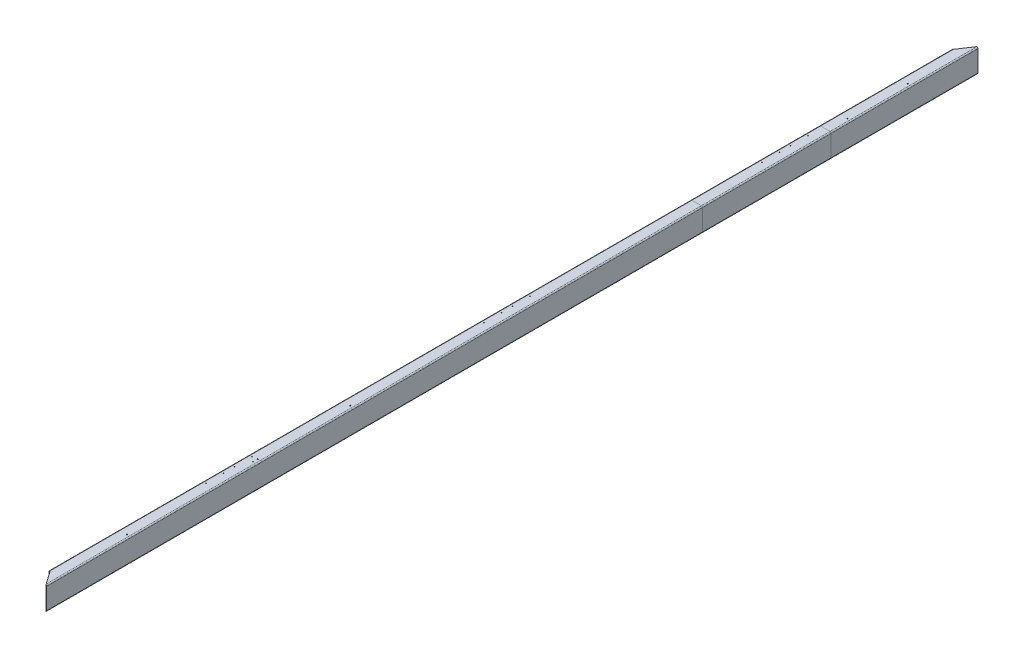
SolidWorks part; units mm, degrees
ref_plane "前视基准面" through (0, 0, 0) normal (0, 0, 1) x (1, 0, 0)
ref_plane "上视基准面" through (0, 0, 0) normal (0, 1, 0) x (1, 0, 0)
ref_plane "右视基准面" through (0, 0, 0) normal (1, 0, 0) x (0, 0, -1)
sketch "草图1" plane through (0, 0, 0) normal (0, 0, 1) x (1, 0, 0)
  line L1 (-20, 50) -> (20, 50)
  line L2 (-25, 45) -> (-25, -45)
  line L3 (-20, -50) -> (20, -50)
  line L4 (25, 45) -> (25, -45)
  line L5 (-25, 50) -> (25, -50) construction
  line L6 (-25, -50) -> (25, 50) construction
  arc A0 (20, -50) -> (25, -45) centre (20, -45) ccw
  arc A1 (-25, -45) -> (-20, -50) centre (-20, -45) ccw
  arc A2 (20, 50) -> (25, 45) centre (20, 45) cw
  arc A3 (-20, 50) -> (-25, 45) centre (-20, 45) ccw
  point P0 (0, 0)
  dimension "D3" = 5
  dimension "D1" = 50
  dimension "D2" = 100
extrude "拉伸-薄壁1" add sketch "草图1" along normal mid plane 2754 thin
sketch "草图2" plane through (0, 0, 1377) normal (0, 0, 1) x (1, 0, 0)
  line L0 (-20, -50) -> (20, -50) construction
  line L1 (-20, -46) -> (20, -46) construction
  line L2 (21, -45) -> (21, 45) construction
  line L3 (25, -45) -> (25, 45) construction
  line L4 (-21, 45) -> (-21, -45) construction
  line L5 (-25, 45) -> (-25, -45) construction
  line L6 (20, 46) -> (-20, 46) construction
  line L7 (20, 50) -> (-20, 50) construction
  line L8 (-20, -50) -> (20, -50)
  line L9 (-20, -46) -> (20, -46)
  line L10 (21, -45) -> (21, 45)
  line L11 (25, -45) -> (25, 45)
  line L12 (-21, 45) -> (-21, -45)
  line L13 (-25, 45) -> (-25, -45)
  line L14 (20, 46) -> (-20, 46)
  line L15 (20, 50) -> (-20, 50)
  arc A0 (20, -50) -> (25, -45) centre (20, -45) ccw construction
  arc A1 (20, -46) -> (21, -45) centre (20, -45) ccw construction
  arc A2 (-25, -45) -> (-20, -50) centre (-20, -45) ccw construction
  arc A3 (-21, -45) -> (-20, -46) centre (-20, -45) ccw construction
  arc A4 (21, 45) -> (20, 46) centre (20, 45) ccw construction
  arc A5 (-20, 46) -> (-21, 45) centre (-20, 45) ccw construction
  arc A6 (25, 45) -> (20, 50) centre (20, 45) ccw construction
  arc A7 (-20, 50) -> (-25, 45) centre (-20, 45) ccw construction
  arc A8 (20, -50) -> (25, -45) centre (20, -45) ccw
  arc A9 (20, -46) -> (21, -45) centre (20, -45) ccw
  arc A10 (-25, -45) -> (-20, -50) centre (-20, -45) ccw
  arc A11 (-21, -45) -> (-20, -46) centre (-20, -45) ccw
  arc A12 (21, 45) -> (20, 46) centre (20, 45) ccw
  arc A13 (-20, 46) -> (-21, 45) centre (-20, 45) ccw
  arc A14 (25, 45) -> (20, 50) centre (20, 45) ccw
  arc A15 (-20, 50) -> (-25, 45) centre (-20, 45) ccw
extrude "凸台-拉伸1" add sketch "草图2" along normal blind 60 separate body
sketch "草图3" plane through (0, 50, 0) normal (0, 1, 0) x (1, 0, 0)
  line L0 (-20, -1377) -> (22.0125, -1437)
  line L2 (20, -1377) -> (-20, -1377) construction
  line L3 (-20, -1377) -> (-44.1333, -1377)
  line L4 (-44.1333, -1377) -> (-44.1333, -1437)
  line L5 (-44.1333, -1437) -> (22.0125, -1437)
  line L6 (20, -1437) -> (-20, -1437) construction
  line L7 (20, -1437) -> (25, -1437) construction
  dimension "D1" = 55
extrude "切除-拉伸1" cut sketch "草图3" against normal through all
sketch "草图4" plane through (0, 0, -1377) normal (0, 0, -1) x (-1, 0, 0)
  line L0 (20, -46) -> (-20, -46) construction
  line L1 (20, -50) -> (-20, -50) construction
  line L2 (-21, -45) -> (-21, 45) construction
  line L3 (-25, -45) -> (-25, 45) construction
  line L4 (25, 45) -> (25, -45) construction
  line L5 (21, 45) -> (21, -45) construction
  line L6 (-20, 46) -> (20, 46) construction
  line L7 (-20, 50) -> (20, 50) construction
  line L8 (20, -46) -> (-20, -46)
  line L9 (20, -50) -> (-20, -50)
  line L10 (-21, -45) -> (-21, 45)
  line L11 (-25, -45) -> (-25, 45)
  line L12 (25, 45) -> (25, -45)
  line L13 (21, 45) -> (21, -45)
  line L14 (-20, 46) -> (20, 46)
  line L15 (-20, 50) -> (20, 50)
  arc A0 (-25, -45) -> (-20, -50) centre (-20, -45) ccw construction
  arc A1 (-21, -45) -> (-20, -46) centre (-20, -45) ccw construction
  arc A2 (20, -46) -> (21, -45) centre (20, -45) ccw construction
  arc A3 (20, -50) -> (25, -45) centre (20, -45) ccw construction
  arc A4 (21, 45) -> (20, 46) centre (20, 45) ccw construction
  arc A5 (25, 45) -> (20, 50) centre (20, 45) ccw construction
  arc A6 (-20, 46) -> (-21, 45) centre (-20, 45) ccw construction
  arc A7 (-20, 50) -> (-25, 45) centre (-20, 45) ccw construction
  arc A8 (-25, -45) -> (-20, -50) centre (-20, -45) ccw
  arc A9 (-21, -45) -> (-20, -46) centre (-20, -45) ccw
  arc A10 (20, -46) -> (21, -45) centre (20, -45) ccw
  arc A11 (20, -50) -> (25, -45) centre (20, -45) ccw
  arc A12 (21, 45) -> (20, 46) centre (20, 45) ccw
  arc A13 (25, 45) -> (20, 50) centre (20, 45) ccw
  arc A14 (-20, 46) -> (-21, 45) centre (-20, 45) ccw
  arc A15 (-20, 50) -> (-25, 45) centre (-20, 45) ccw
extrude "凸台-拉伸2" add sketch "草图4" along normal blind 1182 separate body
sketch "草图5" plane through (0, 50, 0) normal (0, 1, 0) x (1, 0, 0)
  line L0 (20, 2559) -> (-20, 2499)
  line L1 (-20, 2559) -> (-20, 1377) construction
  line L2 (-20, 2559) -> (20, 2559) construction
  line L3 (-20, 2499) -> (-29.878, 2499)
  line L4 (-29.878, 2499) -> (-29.878, 2930.2275)
  line L5 (-29.878, 2930.2275) -> (20, 2930.2275)
  line L6 (20, 2930.2275) -> (20, 2559)
  dimension "D1" = 60
extrude "切除-拉伸2" cut sketch "草图5" against normal through all
sketch "草图6" plane through (0, 50, 0) normal (0, 1, 0) x (1, 0, 0)
  line L0 (-353.4481, 1929) -> (237.5908, 1929)
  line L1 (25, 2559) -> (20, 2559) construction
  dimension "D1" = 630
split line "分割线1"
hole_wizard "M3 螺纹孔1" positions "草图9" profile "草图8" tap size "M3" standard "GB"
sketch "草图9" plane through (0, 50, 0) normal (0, 1, 0) x (1, 0, 0)
  line L1 (-8.25, -717) -> (-13.75, -717) construction
  line L3 (-13.75, -642) -> (-8.25, -642) construction
  line L5 (-13.75, -594.5) -> (-8.25, -594.5) construction
  line L8 (-13.75, -519.5) -> (-8.25, -519.5) construction
  line L10 (-11, -1519.5) -> (-11, 48480.5) construction
  line L11 (-8.25, 476) -> (-11, 476) construction
  line L13 (-8.25, 551) -> (-11, 551) construction
  line L15 (-8.25, 597.5) -> (-11, 597.5) construction
  line L17 (-8.25, 672.5) -> (-11, 672.5) construction
  line L19 (-8.25, 1743) -> (-11, 1743) construction
  line L21 (-8.25, 1668) -> (-11, 1668) construction
  line L23 (-8.25, 1790.5) -> (-11, 1790.5) construction
  line L25 (-8.25, 1865.5) -> (-11, 1865.5) construction
  point P28 (-11, -642)
  point P30 (-11, -717)
  point P32 (-11, -594.5)
  point P34 (-11, -519.5)
  point P44 (-11, 476)
  point P49 (-11, 551)
  point P54 (-11, 597.5)
  point P59 (-11, 672.5)
  point P63 (-11, 1743)
  point P68 (-11, 1668)
  point P72 (-11, 1790.5)
  point P77 (-11, 1865.5)
sketch "草图8" plane through (-11, 50, -1865.5) normal (1, 0, 0) x (0, 0, 1)
  line L0 (0, 0) -> (0, 9.2511)
  line L1 (0, 9.2511) -> (1.25, 8.5)
  line L2 (1.25, 8.5) -> (1.25, 0.275)
  line L3 (1.25, 0.275) -> (1.525, 0)
  line L5 (1.525, 0) -> (0, 0)
  line L6 (-1.25, 0.275) -> (-1.525, 0) construction
  line L10 (0, 9.2511) -> (-1.25, 8.5) construction
  line L11 (0, -6.35) -> (0, 107.95) construction
  dimension "螺纹孔钻头直径" = 2.5
  dimension "螺纹孔钻头深度" = 8.5
  dimension "近端锥形沉头孔直径" = 3.05
  dimension "近端锥形沉头孔角度" = 90
  dimension "导头角度" = 118
cosmetic thread "孔螺蚊线1" parameters "D1"=4, "D2"=3
cosmetic thread "孔螺蚊线2" parameters "D1"=4, "D2"=3
cosmetic thread "孔螺蚊线3" parameters "D1"=4, "D2"=3
cosmetic thread "孔螺蚊线4" parameters "D1"=4, "D2"=3
cosmetic thread "孔螺蚊线5" parameters "D1"=4, "D2"=3
cosmetic thread "孔螺蚊线6" parameters "D1"=4, "D2"=3
cosmetic thread "孔螺蚊线7" parameters "D1"=4, "D2"=3
cosmetic thread "孔螺蚊线8" parameters "D1"=4, "D2"=3
cosmetic thread "孔螺蚊线9" parameters "D1"=4, "D2"=3
cosmetic thread "孔螺蚊线10" parameters "D1"=4, "D2"=3
cosmetic thread "孔螺蚊线11" parameters "D1"=4, "D2"=3
cosmetic thread "孔螺蚊线12" parameters "D1"=4, "D2"=3
hole_wizard "M4 螺纹孔2" positions "草图10" profile "草图11" tap size "M4" standard "GB"
sketch "草图10" plane through (0, 50, 0) normal (0, 1, 0) x (1, 0, 0)
  point P26 (10, -119)
  point P29 (10, -516.4937)
  point P32 (10, -537)
  point P35 (10, -1077)
sketch "草图11" plane through (10, 50, 119) normal (1, 0, 0) x (0, 0, 1)
  line L0 (0, 0) -> (0, 11.0914)
  line L1 (0, 11.0914) -> (1.65, 10.1)
  line L2 (1.65, 10.1) -> (1.65, 0.375)
  line L3 (1.65, 0.375) -> (2.025, 0)
  line L5 (2.025, 0) -> (0, 0)
  line L6 (-1.65, 0.375) -> (-2.025, 0) construction
  line L10 (0, 11.0914) -> (-1.65, 10.1) construction
  line L11 (0, -6.35) -> (0, 107.95) construction
  dimension "螺纹孔钻头直径" = 3.3
  dimension "螺纹孔钻头深度" = 10.1
  dimension "近端锥形沉头孔直径" = 4.05
  dimension "近端锥形沉头孔角度" = 90
  dimension "导头角度" = 118
cosmetic thread "孔螺蚊线13" parameters "D1"=4, "D2"=4
cosmetic thread "孔螺蚊线14" parameters "D1"=4, "D2"=4
cosmetic thread "孔螺蚊线15" parameters "D1"=4, "D2"=4
cosmetic thread "孔螺蚊线16" parameters "D1"=4, "D2"=4
hole_wizard "M4 螺纹孔3" positions "草图12" profile "草图13" tap size "M4" standard "GB"
sketch "草图12" plane through (0, 50, 0) normal (0, 1, 0) x (1, 0, 0)
  point P0 (10, 2014)
sketch "草图13" plane through (10, 50, -2014) normal (1, 0, 0) x (0, 0, 1)
  line L0 (0, 0) -> (0, 11.0914)
  line L1 (0, 11.0914) -> (1.65, 10.1)
  line L2 (1.65, 10.1) -> (1.65, 0.375)
  line L3 (1.65, 0.375) -> (2.025, 0)
  line L5 (2.025, 0) -> (0, 0)
  line L6 (-1.65, 0.375) -> (-2.025, 0) construction
  line L10 (0, 11.0914) -> (-1.65, 10.1) construction
  line L11 (0, -6.35) -> (0, 107.95) construction
  dimension "螺纹孔钻头直径" = 3.3
  dimension "螺纹孔钻头深度" = 10.1
  dimension "近端锥形沉头孔直径" = 4.05
  dimension "近端锥形沉头孔角度" = 90
  dimension "导头角度" = 118
cosmetic thread "孔螺蚊线17" parameters "D1"=4, "D2"=4
combine bodies "组合1" operation type add bodies to combine 103 110
sketch "草图14" plane through (0, 50, 0) normal (0, 1, 0) x (1, 0, 0)
  line L0 (25, 2559) -> (20, 2559) construction
  line L1 (25, 2559) -> (25, 1929) construction
  circle A0 centre (10, 2272.7) radius 1.65
  dimension "D1" = 3.3
  dimension "D2" = 286.3
  dimension "D3" = 15
extrude "切除-拉伸3" cut sketch "草图14" against normal blind 10
cosmetic thread "装饰螺纹线1" parameters "D2"=4
